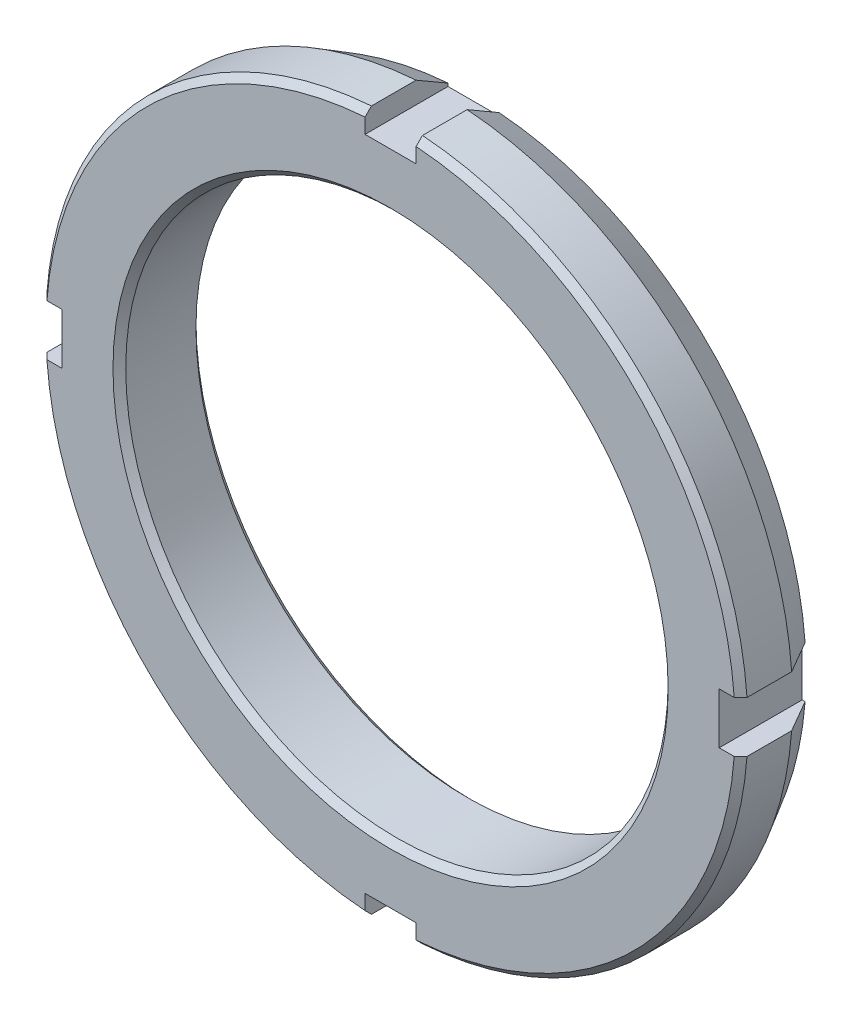
from build123d import *
from OCP.BRepFilletAPI import BRepFilletAPI_MakeChamfer

# Parameters (mm, degrees)
SKETCH2_R           = 110
BOSS_EXTRUDE1_DEPTH = 26
CUT_EXTRUDE1_DEPTH  = 26
CHAMFER1_SIZE       = 2
CHAMFER2_SIZE       = 10
CHAMFER2_SIZE2      = 5.773502692
SKETCH4_R           = 85
CUT_EXTRUDE2_DEPTH  = 26
CHAMFER3_SIZE       = 2


with BuildPart() as part:
    # Sketch2 → Boss-Extrude1 (new body)
    with BuildSketch(Plane.XY):
        with Locations(Location((0, 0, 0), (0, 0, 180))):
            Circle(SKETCH2_R)
    extrude(amount=BOSS_EXTRUDE1_DEPTH)

    # Sketch3 → Cut-Extrude1 (cut)
    with BuildSketch(Plane.XY.offset(26)):
        with BuildLine():
            Line((-8, 109.954040528), (-8, 103))
            Line((-8, 103), (8, 103))
            Line((8, 103), (8, 109.954040528))
            ThreePointArc((8, 109.954040528), (0, 110.244687076), (-8, 109.954040528))
        make_face()
        with BuildLine():
            Line((-109.954040528, -8), (-103, -8))
            Line((-103, -8), (-103, 8))
            Line((-103, 8), (-109.954040528, 8))
            ThreePointArc((-109.954040528, 8), (-110.244687076, 0), (-109.954040528, -8))
        make_face()
        with BuildLine():
            Line((103, 8), (103, -8))
            Line((103, -8), (109.954040528, -8))
            ThreePointArc((109.954040528, -8), (110.244687076, 0), (109.954040528, 8))
            Line((109.954040528, 8), (103, 8))
        make_face()
        with BuildLine():
            Line((-8, -103), (-8, -109.954040528))
            ThreePointArc((-8, -109.954040528), (0, -110.244687076), (8, -109.954040528))
            Line((8, -109.954040528), (8, -103))
            Line((8, -103), (-8, -103))
        make_face()
    extrude(amount=-CUT_EXTRUDE1_DEPTH, mode=Mode.SUBTRACT)

    # Chamfer1
    chamfer1_edges = [part.edges().sort_by_distance(p)[0] for p in [
        (-77.781745931, 77.781745931, 26),
        (77.781745931, 77.781745931, 26),
        (-77.781745931, -77.781745931, 26),
        (77.781745931, -77.781745931, 26),
    ]]
    chamfer(chamfer1_edges, length=CHAMFER1_SIZE)

    # Chamfer2: one chamfer whose edges measure the first distance from different faces: ONE call of the kernel's chamfer builder (chamfer() names one face for all edges)
    chamfer2_edges_1 = [part.edges().sort_by_distance(p)[0] for p in [
        (77.781745931, 77.781745931, 0),
    ]]
    chamfer2_side_1 = [part.faces().sort_by_distance(p)[0] for p in [
        (77.781745931, 77.781745931, 12),
    ]]
    chamfer2_edges_2 = [part.edges().sort_by_distance(p)[0] for p in [
        (-77.781745931, 77.781745931, 0),
    ]]
    chamfer2_side_2 = [part.faces().sort_by_distance(p)[0] for p in [
        (-77.781745931, 77.781745931, 12),
    ]]
    chamfer2_edges_3 = [part.edges().sort_by_distance(p)[0] for p in [
        (-77.781745931, -77.781745931, 0),
    ]]
    chamfer2_side_3 = [part.faces().sort_by_distance(p)[0] for p in [
        (-77.781745931, -77.781745931, 12),
    ]]
    chamfer2_edges_4 = [part.edges().sort_by_distance(p)[0] for p in [
        (77.781745931, -77.781745931, 0),
    ]]
    chamfer2_side_4 = [part.faces().sort_by_distance(p)[0] for p in [
        (77.781745931, -77.781745931, 12),
    ]]
    chamfer2 = BRepFilletAPI_MakeChamfer(part.part.solid().wrapped)
    for e in chamfer2_edges_1:
        chamfer2.Add(CHAMFER2_SIZE, CHAMFER2_SIZE2, e.wrapped, chamfer2_side_1[0].wrapped)  # the first distance lies on this face
    for e in chamfer2_edges_2:
        chamfer2.Add(CHAMFER2_SIZE, CHAMFER2_SIZE2, e.wrapped, chamfer2_side_2[0].wrapped)  # the first distance lies on this face
    for e in chamfer2_edges_3:
        chamfer2.Add(CHAMFER2_SIZE, CHAMFER2_SIZE2, e.wrapped, chamfer2_side_3[0].wrapped)  # the first distance lies on this face
    for e in chamfer2_edges_4:
        chamfer2.Add(CHAMFER2_SIZE, CHAMFER2_SIZE2, e.wrapped, chamfer2_side_4[0].wrapped)  # the first distance lies on this face
    add(Compound.cast(chamfer2.Shape()), mode=Mode.REPLACE)

    # Sketch4 → Cut-Extrude2 (cut)
    with BuildSketch(Plane(origin=(0, 0, 0), x_dir=(-1, 0, 0), z_dir=(0, 0, -1))):
        Circle(SKETCH4_R)
    extrude(amount=-CUT_EXTRUDE2_DEPTH, mode=Mode.SUBTRACT)

    # Chamfer3
    chamfer3_edges = [part.edges().sort_by_distance(p)[0] for p in [
        (85, 0, 26),
        (85, 0, 0),
    ]]
    chamfer(chamfer3_edges, length=CHAMFER3_SIZE)


solid = part.part
